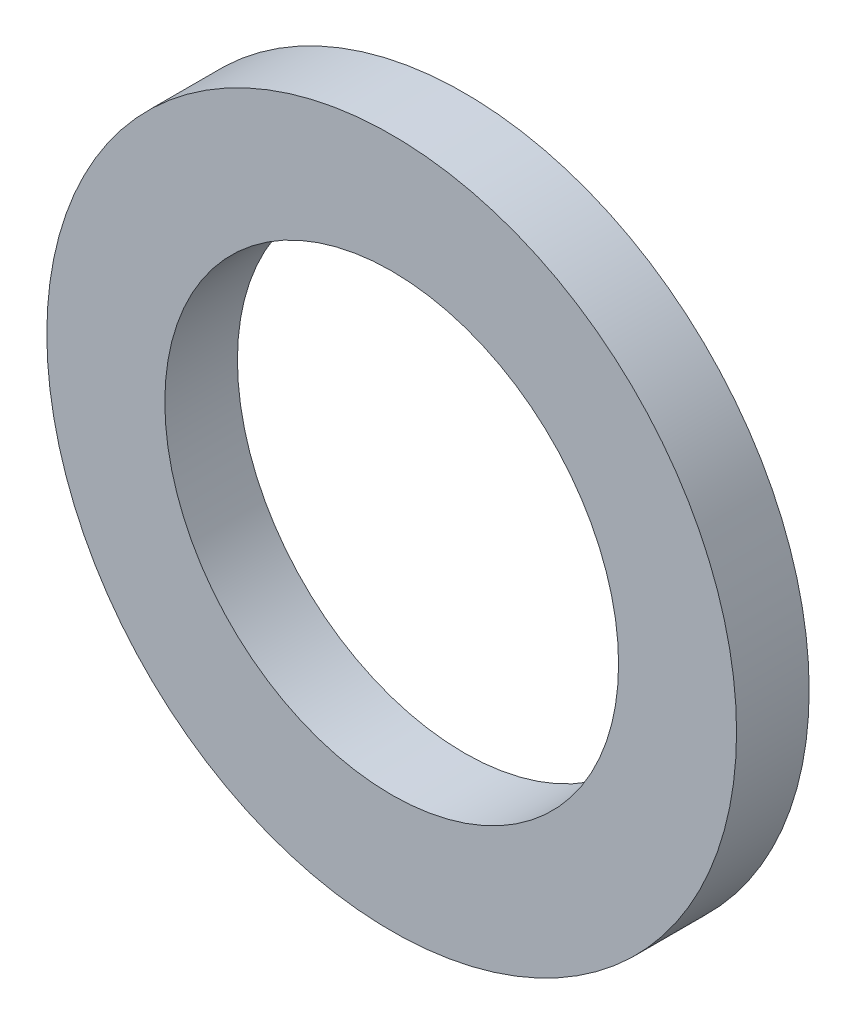
from build123d import *

# Parameters (mm, degrees)
SKETCH1_R      = 19
SKETCH1_R_2    = 12.5
EXTRUDE1_DEPTH = 4


with BuildPart() as part:
    # Sketch1 → Extrude1 (new body)
    with BuildSketch(Plane.XY):
        Circle(SKETCH1_R)
        Circle(SKETCH1_R_2, mode=Mode.SUBTRACT)
    extrude(amount=EXTRUDE1_DEPTH)


solid = part.part
